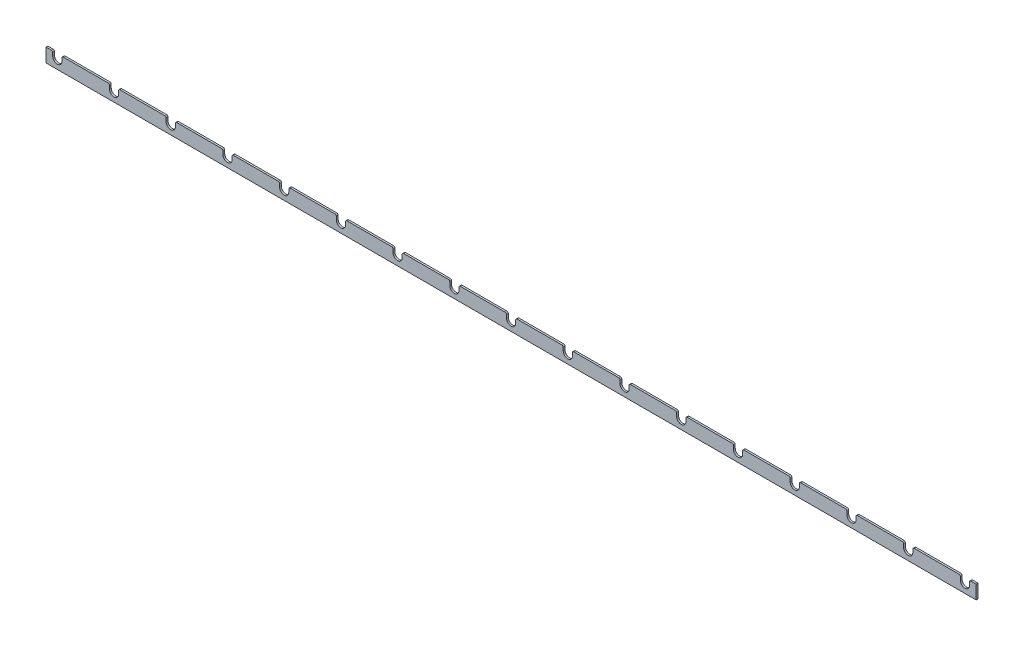
SolidWorks part; units mm, degrees
ref_plane "前视基准面" through (0, 0, 0) normal (0, 0, 1) x (1, 0, 0)
ref_plane "上视基准面" through (0, 0, 0) normal (0, 1, 0) x (1, 0, 0)
ref_plane "右视基准面" through (0, 0, 0) normal (1, 0, 0) x (0, 0, -1)
sketch "草图1" plane through (0, 0, 0) normal (0, 0, 1) x (1, 0, 0)
  line L1 (1015, 15) -> (-1015, 15)
  line L2 (1015, 15) -> (1015, -15)
  line L3 (1015, -15) -> (-1015, -15)
  line L4 (-1015, 15) -> (-1015, -15)
  line L5 (1015, 15) -> (-1015, -15) construction
  line L6 (1015, -15) -> (-1015, 15) construction
  point P0 (0, 0)
  dimension "D1" = 2030
  dimension "D2" = 30
extrude "凸台-拉伸1" add sketch "草图1" along normal blind 4
sketch "草图2" plane through (0, 0, 4) normal (0, 0, 1) x (1, 0, 0)
  line L0 (1015, 15) -> (-1015, 15) construction
  line L1 (-1000.4, 5) -> (-980.4, 5) construction
  line L2 (-1015, 15) -> (-1015, -15) construction
  line L3 (-1000.4, 5) -> (-1000.4, 15)
  line L4 (-980.4, 5) -> (-980.4, 15)
  line L5 (-980.4, 15) -> (-1000.4, 15)
  line L6 (-856.6, 15) -> (-876.6, 15)
  line L7 (-876.6, 5) -> (-876.6, 15)
  line L8 (-856.6, 5) -> (-856.6, 15)
  line L9 (-732.8, 15) -> (-752.8, 15)
  line L10 (-752.8, 5) -> (-752.8, 15)
  line L11 (-732.8, 5) -> (-732.8, 15)
  line L12 (-609, 15) -> (-629, 15)
  line L13 (-629, 5) -> (-629, 15)
  line L14 (-609, 5) -> (-609, 15)
  line L15 (-485.2, 15) -> (-505.2, 15)
  line L16 (-505.2, 5) -> (-505.2, 15)
  line L17 (-485.2, 5) -> (-485.2, 15)
  line L18 (-361.4, 15) -> (-381.4, 15)
  line L19 (-381.4, 5) -> (-381.4, 15)
  line L20 (-361.4, 5) -> (-361.4, 15)
  line L21 (-237.6, 15) -> (-257.6, 15)
  line L22 (-257.6, 5) -> (-257.6, 15)
  line L23 (-237.6, 5) -> (-237.6, 15)
  line L24 (-113.8, 15) -> (-133.8, 15)
  line L25 (-133.8, 5) -> (-133.8, 15)
  line L26 (-113.8, 5) -> (-113.8, 15)
  line L27 (10, 15) -> (-10, 15)
  line L28 (-10, 5) -> (-10, 15)
  line L29 (10, 5) -> (10, 15)
  line L30 (133.8, 15) -> (113.8, 15)
  line L31 (113.8, 5) -> (113.8, 15)
  line L32 (133.8, 5) -> (133.8, 15)
  line L33 (257.6, 15) -> (237.6, 15)
  line L34 (237.6, 5) -> (237.6, 15)
  line L35 (257.6, 5) -> (257.6, 15)
  line L36 (381.4, 15) -> (361.4, 15)
  line L37 (361.4, 5) -> (361.4, 15)
  line L38 (381.4, 5) -> (381.4, 15)
  line L39 (505.2, 15) -> (485.2, 15)
  line L40 (485.2, 5) -> (485.2, 15)
  line L41 (505.2, 5) -> (505.2, 15)
  line L42 (629, 15) -> (609, 15)
  line L43 (609, 5) -> (609, 15)
  line L44 (629, 5) -> (629, 15)
  line L45 (752.8, 15) -> (732.8, 15)
  line L46 (732.8, 5) -> (732.8, 15)
  line L47 (752.8, 5) -> (752.8, 15)
  line L48 (876.6, 15) -> (856.6, 15)
  line L49 (856.6, 5) -> (856.6, 15)
  line L50 (876.6, 5) -> (876.6, 15)
  line L51 (1000.4, 15) -> (980.4, 15)
  line L52 (980.4, 5) -> (980.4, 15)
  line L53 (1000.4, 5) -> (1000.4, 15)
  arc A0 (-996.9, 5) -> (-983.9, 5) centre (-990.4, 5) ccw construction
  arc A1 (-1000.4, 5) -> (-980.4, 5) centre (-990.4, 5) ccw
  arc A2 (-876.6, 5) -> (-856.6, 5) centre (-866.6, 5) ccw
  arc A3 (-752.8, 5) -> (-732.8, 5) centre (-742.8, 5) ccw
  arc A4 (-629, 5) -> (-609, 5) centre (-619, 5) ccw
  arc A5 (-505.2, 5) -> (-485.2, 5) centre (-495.2, 5) ccw
  arc A6 (-381.4, 5) -> (-361.4, 5) centre (-371.4, 5) ccw
  arc A7 (-257.6, 5) -> (-237.6, 5) centre (-247.6, 5) ccw
  arc A8 (-133.8, 5) -> (-113.8, 5) centre (-123.8, 5) ccw
  arc A9 (-10, 5) -> (10, 5) centre (0, 5) ccw
  arc A10 (113.8, 5) -> (133.8, 5) centre (123.8, 5) ccw
  arc A11 (237.6, 5) -> (257.6, 5) centre (247.6, 5) ccw
  arc A12 (361.4, 5) -> (381.4, 5) centre (371.4, 5) ccw
  arc A13 (485.2, 5) -> (505.2, 5) centre (495.2, 5) ccw
  arc A14 (609, 5) -> (629, 5) centre (619, 5) ccw
  arc A15 (732.8, 5) -> (752.8, 5) centre (742.8, 5) ccw
  arc A16 (856.6, 5) -> (876.6, 5) centre (866.6, 5) ccw
  arc A17 (980.4, 5) -> (1000.4, 5) centre (990.4, 5) ccw
  dimension "D2" = 13
  dimension "D3" = 20
  dimension "D4" = 24.6
  dimension "D1" = 10
  dimension "D5" = 17
extrude "切除-拉伸1" cut sketch "草图2" against normal blind 4
fillet "圆角1" radius 3 34 edges at (980.4, 15, 2) (1000.4, 15, 2) (856.6, 15, 2) (876.6, 15, 2) (732.8, 15, 2) (752.8, 15, 2) (609, 15, 2) (629, 15, 2) (485.2, 15, 2) (505.2, 15, 2) (361.4, 15, 2) (381.4, 15, 2) (237.6, 15, 2) (257.6, 15, 2) (113.8, 15, 2) (133.8, 15, 2) (-10, 15, 2) (10, 15, 2) (-133.8, 15, 2) (-113.8, 15, 2) (-257.6, 15, 2) (-237.6, 15, 2) (-381.4, 15, 2) (-361.4, 15, 2) (-505.2, 15, 2) (-485.2, 15, 2) (-629, 15, 2) (-609, 15, 2) (-752.8, 15, 2) (-732.8, 15, 2) (-876.6, 15, 2) (-856.6, 15, 2) (-1000.4, 15, 2) (-980.4, 15, 2)
